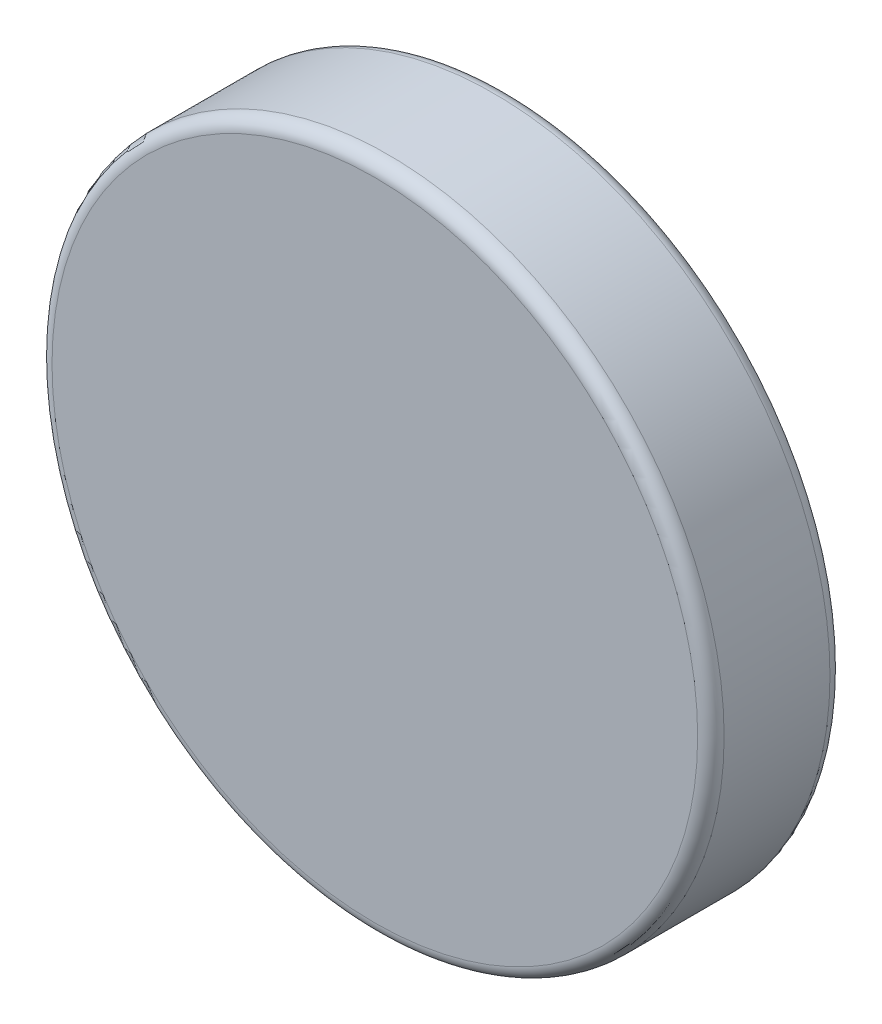
SolidWorks part; units mm, degrees
ref_plane "Front Plane" through (0, 0, 0) normal (0, 0, 1) x (1, 0, 0)
ref_plane "Top Plane" through (0, 0, 0) normal (0, 1, 0) x (1, 0, 0)
ref_plane "Right Plane" through (0, 0, 0) normal (1, 0, 0) x (0, 0, -1)
other "Configuration Table"
sketch "Sketch1" plane through (0, 0, 0) normal (0, 0, 1) x (1, 0, 0)
  circle A0 centre (0, 0) radius 12.7
  dimension "D1" = 25.4
extrude "Boss-Extrude1" add sketch "Sketch1" along normal blind 5
fillet "Fillet1" radius 0.5 2 edges at (12.7, 0, 0) (12.7, 0, 5)
